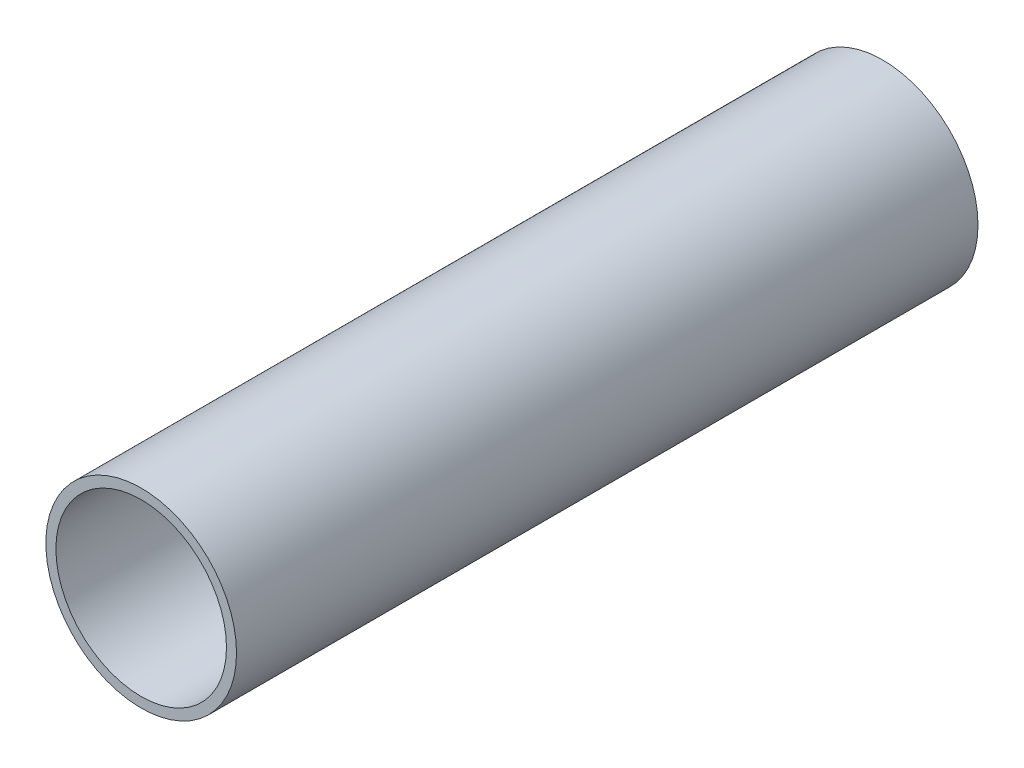
from build123d import *

# Parameters (mm, degrees)
BOSS_EXTRUDE1_DEPTH      = 222.25
BOSS_EXTRUDE1_DEPTH_BACK = 222.25
SKETCH1_R                = 57.15
SKETCH1_R_2              = 51.1302


with BuildPart() as part:
    # Sketch1 → Boss-Extrude1 (new, two sides: drawn at the far end of the back side and taken through both)
    with BuildSketch(Plane.XY.offset(-BOSS_EXTRUDE1_DEPTH_BACK)):
        Circle(SKETCH1_R)
        Circle(SKETCH1_R_2, mode=Mode.SUBTRACT)
    extrude(amount=BOSS_EXTRUDE1_DEPTH + BOSS_EXTRUDE1_DEPTH_BACK)


solid = part.part
